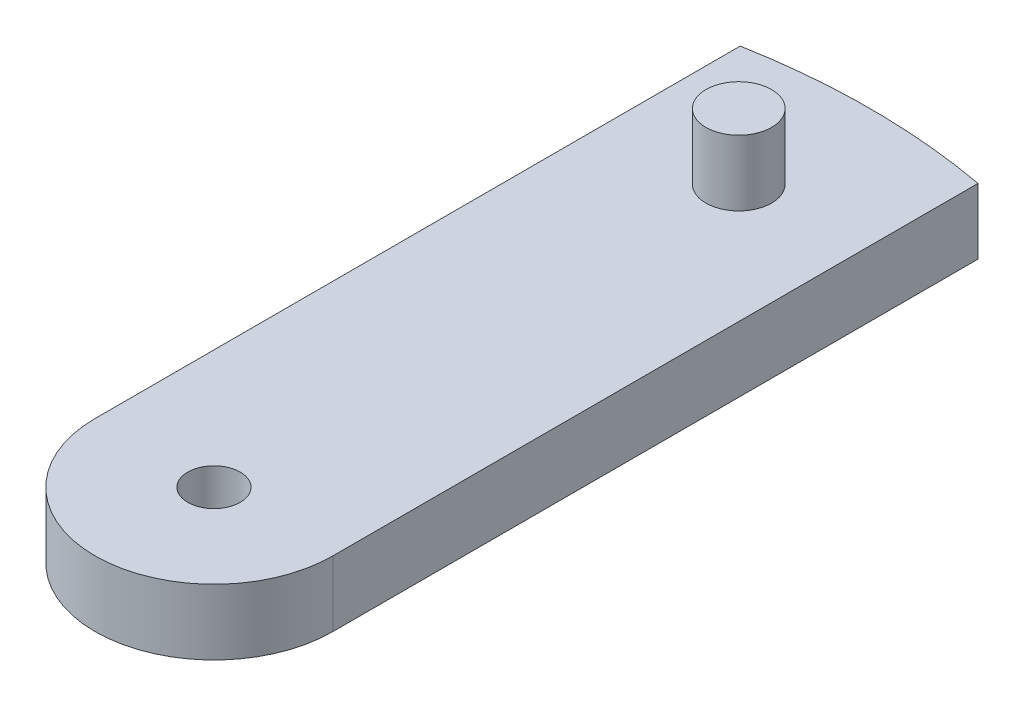
from build123d import *

# Parameters (mm, degrees)
SKETCH_1_3_R        = 50
SKETCH_1_3_R_2      = 2.5
BOSS_EXTRUDE1_DEPTH = 5
SKETCH_1_3_2_R      = 2.5
BOSS_EXTRUDE2_DEPTH = 10
CUT_EXTRUDE1_START  = -11
CUT_EXTRUDE1_DEPTH  = 11
SKETCH2_R           = 2
CUT_EXTRUDE2_DEPTH  = 52.789634215


with BuildPart() as part:
    # Sketch 1_3 → Boss-Extrude1 (new body)
    # profile 1 of 2: a face of its own
    with BuildSketch(Plane(origin=(0, 0, 0), x_dir=(1, 0, 0), z_dir=(0, 1, 0))):
        with Locations(Location((0, 0, 0), (0, 0, 270))):
            Circle(SKETCH_1_3_R)
        with Locations((0, 40)):
            Circle(SKETCH_1_3_R_2, mode=Mode.SUBTRACT)
    # profile 2 of 2: a face of its own
    with BuildSketch(Plane(origin=(0, 0, 0), x_dir=(1, 0, 0), z_dir=(0, 1, 0))):
        with Locations((0, 40)):
            Circle(SKETCH_1_3_R_2)
    extrude(amount=BOSS_EXTRUDE1_DEPTH)

    # Sketch 1_3 2 → Boss-Extrude2 (add)
    with BuildSketch(Plane(origin=(0, 0, 0), x_dir=(1, 0, 0), z_dir=(0, 1, 0))):
        with Locations(Location((0, 40, 0), (0, 0, 270))):
            Circle(SKETCH_1_3_2_R)
    extrude(amount=BOSS_EXTRUDE2_DEPTH)

    # Sketch5 → Cut-Extrude1 (cut)
    with BuildSketch(Plane(origin=(0, 5, 0), x_dir=(1, 0, 0), z_dir=(0, 1, 0)).offset(CUT_EXTRUDE1_START)):
        with BuildLine():
            Line((9.064558023, 20), (9.064558023, 0))
            ThreePointArc((9.064558023, 0), (0, -9.064558023), (-9.064558023, 0))
            Line((-9.064558023, 0), (-9.064558023, 20))
            Line((-9.064558023, 20), (-9.064558023, 49.171473314))
            ThreePointArc((-9.064558023, 49.171473314), (0, -50), (9.064558023, 49.171473314))
            Line((9.064558023, 49.171473314), (9.064558023, 20))
        make_face()
    extrude(amount=CUT_EXTRUDE1_DEPTH, mode=Mode.SUBTRACT)

    # Sketch2 → Cut-Extrude2 (cut, through all)
    with BuildSketch(Plane.XZ):
        with Locations(Location((0, 0, 0), (0, 0, 270))):
            Circle(SKETCH2_R)
    extrude(amount=-CUT_EXTRUDE2_DEPTH, mode=Mode.SUBTRACT)


solid = part.part
